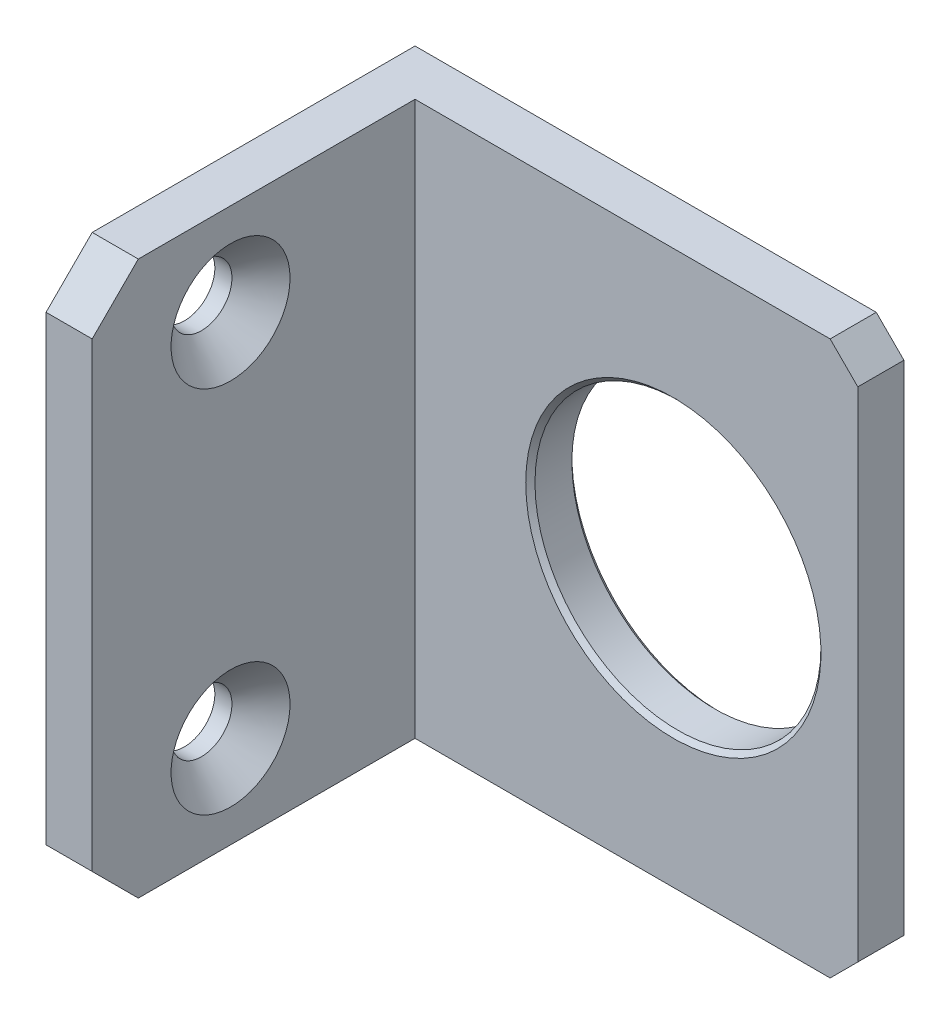
SolidWorks part; units mm, degrees
material "A6061"
ref_plane "前基準面" through (0, 0, 0) normal (0, 0, 1) x (1, 0, 0)
ref_plane "上基準面" through (0, 0, 0) normal (0, 1, 0) x (1, 0, 0)
ref_plane "右基準面" through (0, 0, 0) normal (1, 0, 0) x (0, 0, -1)
sketch "草图1" plane through (0, 0, 0) normal (0, 1, 0) x (1, 0, 0)
  line L0 (0, 0) -> (0, 40)
  line L1 (0, 40) -> (53, 40)
  line L2 (5, 0) -> (5, 35)
  line L3 (5, 35) -> (53, 35)
  line L4 (53, 40) -> (53, 35)
  line L5 (5, 0) -> (0, 0)
  dimension "D1" = 40
  dimension "D2" = 53
  dimension "D3" = 5
extrude "凸台-拉伸1" add sketch "草图1" along normal blind 60
sketch "草图2" plane through (0, 0, -40) normal (0, 0, -1) x (-1, 0, 0)
  line L0 (-53, 60) -> (-53, 0) construction
  circle A0 centre (-33, 30) radius 15.5
  point P4 (-53, 30)
  dimension "D1" = 31
  dimension "D2" = 20
extrude "切除-拉伸1" cut sketch "草图2" against normal through all
chamfer "倒角1" distance 3 angle 45 2 edges at (53, 60, -37.5) (53, 0, -37.5)
chamfer "倒角2" distance 5 angle 45 2 edges at (2.5, 0, 0) (2.5, 60, 0)
hole_wizard "打孔尺寸根据十字槽沉头木螺钉的类型1" positions "草图4" profile "草图3" countersink size "M6" standard "GB" end condition through all
sketch "草图4" plane through (5, 0, 0) normal (1, 0, 0) x (0, 0, -1)
  line L0 (35, 30) -> (-10.4108, 30) construction
  line L1 (35, 60) -> (35, 0) construction
  line L2 (0, 55) -> (0, 5) construction
  line L3 (5, 0) -> (35, 0) construction
  point P0 (15, 10)
  point P7 (15, 50)
  dimension "D1" = 40
  dimension "D2" = 15
  dimension "D3" = 30
sketch "草图3" plane through (5, 10, -15) normal (0, 1, 0) x (0, 0, -1)
  line L0 (0, 0) -> (0, 5)
  line L1 (0, 5) -> (3.3, 5)
  line L2 (3.3, 5) -> (3.3, 3.15)
  line L3 (3.3, 3.15) -> (6.45, 0)
  line L5 (6.45, 0) -> (0, 0)
  line L6 (-3.3, 3.15) -> (-6.45, 0) construction
  line L11 (0, -6.35) -> (0, 107.95) construction
  dimension "通孔孔直径" = 6.6
  dimension "通孔孔深度" = 5
  dimension "近端锥形沉头孔直径" = 12.9
  dimension "近端锥形沉头孔角度" = 90
chamfer "倒角3" distance 0.5 angle 45 2 edges at (17.5, 30, -40) (17.5, 30, -35)
